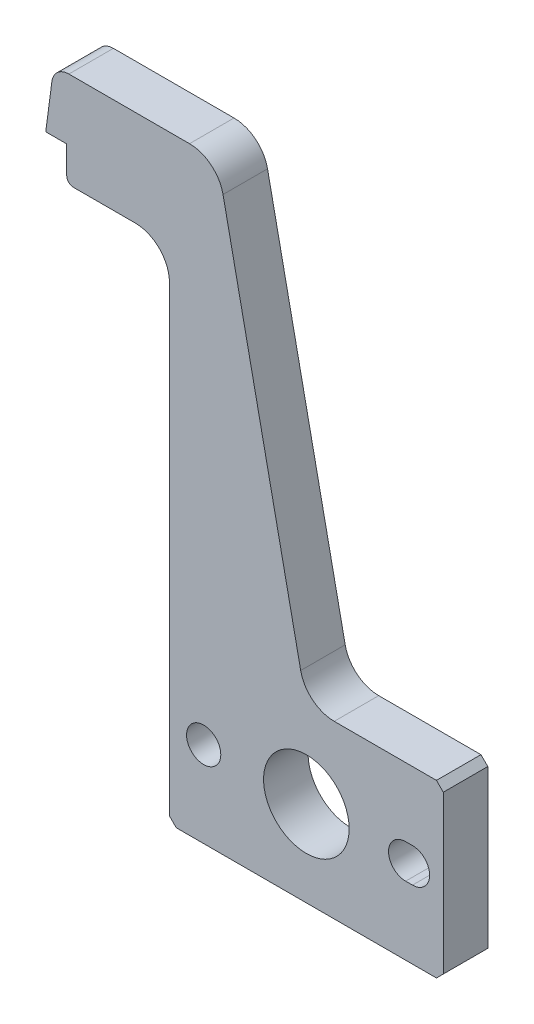
from build123d import *

# Parameters (mm, degrees)
SKETCH1_W           = 11.6
SKETCH1_H           = 17.5
BOSS_EXTRUDE1_DEPTH = 0.65
SKETCH2_R           = 1.25
SKETCH2_R_2         = 0.5
CUT_EXTRUDE1_DEPTH  = 11.577925127
SKETCH3_W           = 3.6
SKETCH3_H           = 14.7
CUT_EXTRUDE2_DEPTH  = 11.577925127
SKETCH4_W           = 0.6
SKETCH4_H           = 1
CUT_EXTRUDE3_DEPTH  = 11.577925127
FILLET2_R           = 0.2
CUT_EXTRUDE4_DEPTH  = 11.577925127
FILLET3_R           = 1
CHAMFER1_SIZE       = 0.2
FILLET4_R           = 0.5


with BuildPart() as part:
    # Sketch1 → Boss-Extrude1 (new, symmetric)
    with BuildSketch(Plane.XY):
        Rectangle(SKETCH1_W, SKETCH1_H)
    extrude(amount=BOSS_EXTRUDE1_DEPTH, both=True)

    # Sketch2 → Cut-Extrude1 (cut, through all)
    with BuildSketch(Plane.XY.offset(0.65)):
        with Locations((1.8, -6.25)):
            Circle(SKETCH2_R)
        with Locations((-1.2, -6.25)):
            Circle(SKETCH2_R_2)
        with BuildLine():
            Line((4.7, -5.75), (4.9, -5.75))
            ThreePointArc((4.9, -5.75), (5.4, -6.25), (4.9, -6.75))
            Line((4.9, -6.75), (4.7, -6.75))
            ThreePointArc((4.7, -6.75), (4.2, -6.25), (4.7, -5.75))
        make_face()
    extrude(amount=-CUT_EXTRUDE1_DEPTH, mode=Mode.SUBTRACT)

    # Sketch3 → Cut-Extrude2 (cut, through all)
    with BuildSketch(Plane.XY.offset(0.65)):
        with Locations((-4, -1.4)):
            Rectangle(SKETCH3_W, SKETCH3_H)
        Polygon((5.8, -3.75), (1.8, -3.75), (-0.8, 8.75), (5.8, 8.75), align=None)
    extrude(amount=-CUT_EXTRUDE2_DEPTH, mode=Mode.SUBTRACT)

    # Sketch4 → Cut-Extrude3 (cut, through all)
    with BuildSketch(Plane.XY.offset(0.65)):
        with Locations((-5.5, 6.45)):
            Rectangle(SKETCH4_W, SKETCH4_H)
    extrude(amount=-CUT_EXTRUDE3_DEPTH, mode=Mode.SUBTRACT)

    # Fillet2
    fillet2_edges = [part.edges().sort_by_distance(p)[0] for p in [
        (-5.2, 5.95, 0),
    ]]
    fillet(fillet2_edges, radius=FILLET2_R)

    # Sketch5 → Cut-Extrude4 (cut, through all)
    with BuildSketch(Plane.XY.offset(0.65)):
        Polygon((-5.8, 7.05), (-5.576190754, 8.75), (-5.8, 8.75), align=None)
    extrude(amount=-CUT_EXTRUDE4_DEPTH, mode=Mode.SUBTRACT)

    # Fillet3
    fillet3_edges = [part.edges().sort_by_distance(p)[0] for p in [
        (-2.2, 5.95, 0),
        (1.8, -3.75, 0),
        (-0.8, 8.75, 0),
    ]]
    fillet(fillet3_edges, radius=FILLET3_R)

    # Chamfer1
    chamfer1_edges = [part.edges().sort_by_distance(p)[0] for p in [
        (-2.2, -8.75, 0),
        (5.8, -3.75, 0),
        (5.8, -8.75, 0),
    ]]
    chamfer(chamfer1_edges, length=CHAMFER1_SIZE)

    # Fillet4
    fillet4_edges = [part.edges().sort_by_distance(p)[0] for p in [
        (-5.576190754, 8.75, 0),
    ]]
    fillet(fillet4_edges, radius=FILLET4_R)


solid = part.part
